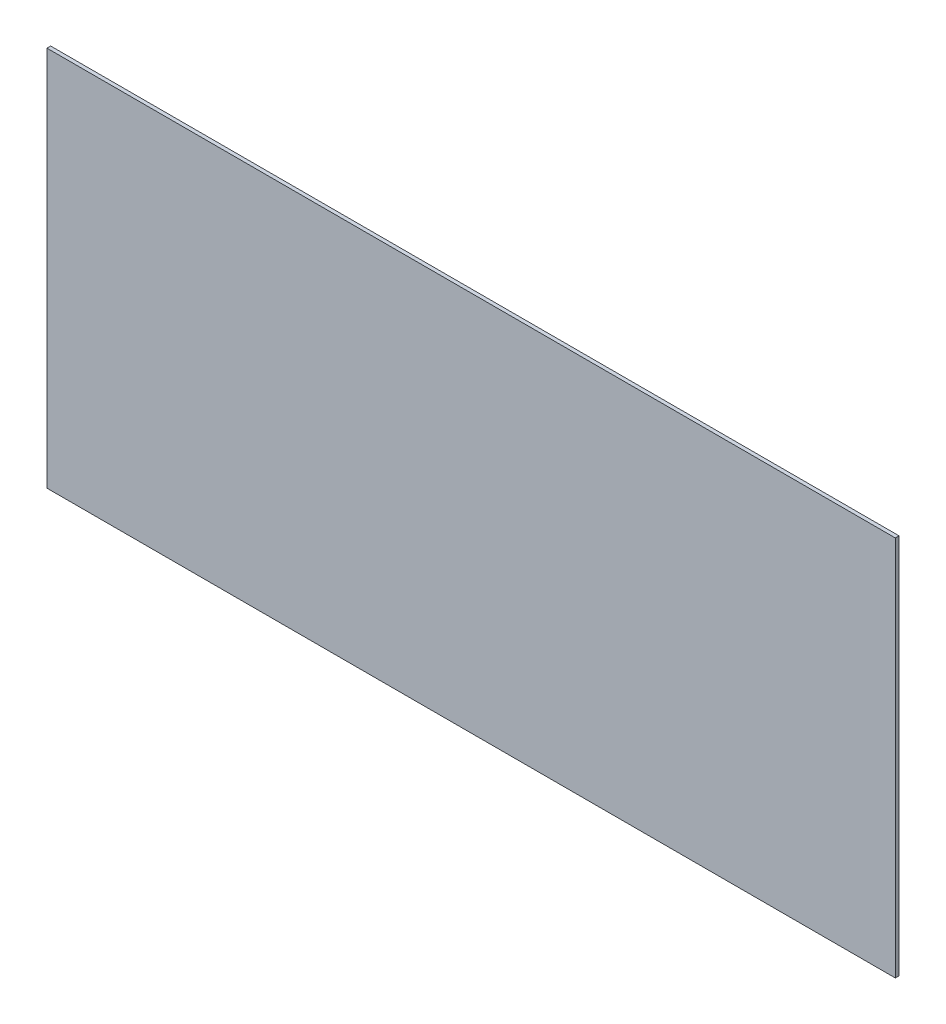
from build123d import *

# Parameters (mm, degrees)
SKETCH_1_W      = 1142
SKETCH_1_H      = 513
EXTRUDE_1_DEPTH = 5


with BuildPart() as part:
    # 草图1 → 凸台-拉伸1 (new body)
    with BuildSketch(Plane.XY):
        Rectangle(SKETCH_1_W, SKETCH_1_H)
    extrude(amount=EXTRUDE_1_DEPTH)


solid = part.part
